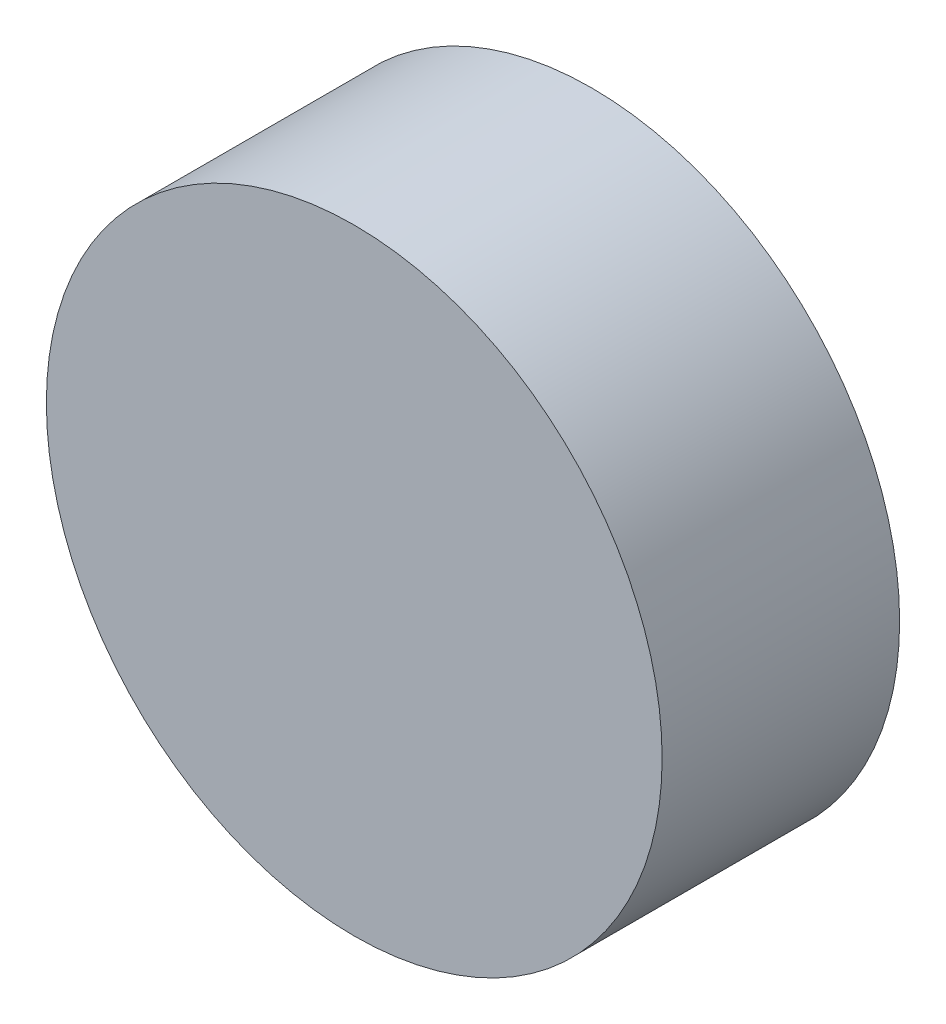
SolidWorks part; units mm, degrees
ref_plane "Front Plane" through (0, 0, 0) normal (0, 0, 1) x (1, 0, 0)
ref_plane "Top Plane" through (0, 0, 0) normal (0, 1, 0) x (1, 0, 0)
ref_plane "Right Plane" through (0, 0, 0) normal (1, 0, 0) x (0, 0, -1)
sketch "Sketch1" plane through (0, 0, 0) normal (0, 0, 1) x (1, 0, 0)
  circle A0 centre (-17.0558, 0) radius 12.9635
extrude "Boss-Extrude1" add sketch "Sketch1" along normal blind 10
